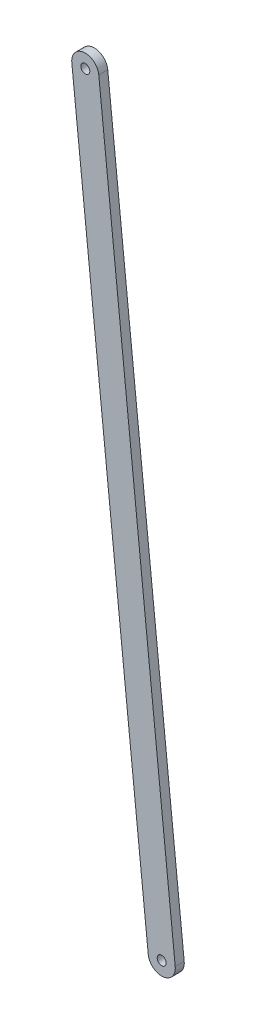
from build123d import *

# Parameters (mm, degrees)
SKETCH3_R           = 5
BOSS_EXTRUDE1_DEPTH = 10


with BuildPart() as part:
    # Sketch3 → Boss-Extrude1 (new body)
    with BuildSketch(Plane.XY):
        with BuildLine():
            Line((-15, 796.465754902), (70, -19.802144846))
            ThreePointArc((70, -19.802144846), (86.561987186, -33.24015766), (100, -16.678170473))
            Line((100, -16.678170473), (15, 799.589729274))
            ThreePointArc((15, 799.589729274), (-1.561987186, 813.027742088), (-15, 796.465754902))
        make_face()
        with Locations((0, 798.027742088)):
            Circle(SKETCH3_R, mode=Mode.SUBTRACT)
        with Locations((85, -18.24015766)):
            Circle(SKETCH3_R, mode=Mode.SUBTRACT)
    extrude(amount=BOSS_EXTRUDE1_DEPTH)


solid = part.part
